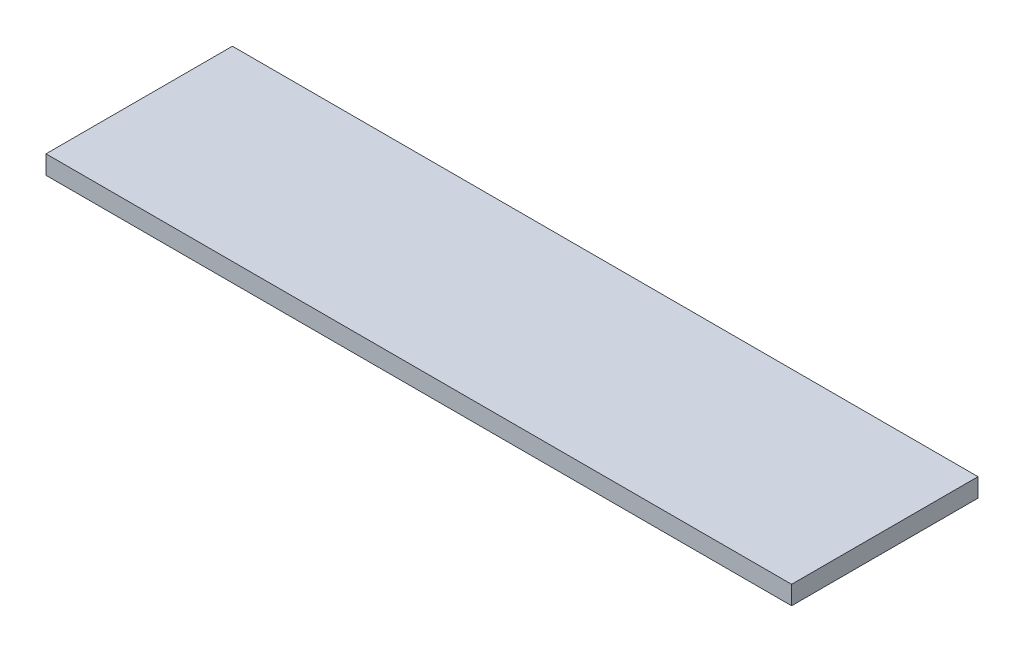
from build123d import *

# Parameters (mm, degrees)
SKETCH1_W      = 1000
SKETCH1_H      = 250
EXTRUDE1_DEPTH = 12.5


with BuildPart() as part:
    # Sketch1 → Extrude1 (new, symmetric)
    with BuildSketch(Plane(origin=(0, 0, 0), x_dir=(1, 0, 0), z_dir=(0, 1, 0))):
        Rectangle(SKETCH1_W, SKETCH1_H)
    extrude(amount=EXTRUDE1_DEPTH, both=True)


solid = part.part
